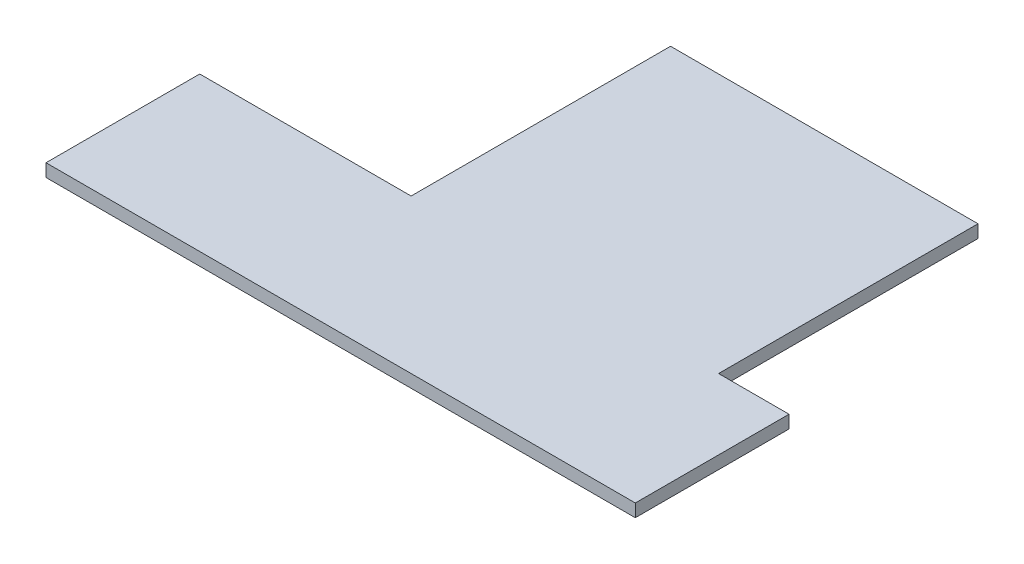
from build123d import *

# Parameters (mm, degrees)
BOSS_EXTRUDE1_DEPTH = 20


with BuildPart() as part:
    # Sketch1 → Boss-Extrude1 (new body)
    with BuildSketch(Plane(origin=(0, 0, 0), x_dir=(1, 0, 0), z_dir=(0, 1, 0))):
        Polygon((-330, -655), (590, -655), (590, -415), (480, -415), (480, -10), (0, -10), (0, -415), (-330, -415), align=None)
    extrude(amount=BOSS_EXTRUDE1_DEPTH)


solid = part.part
